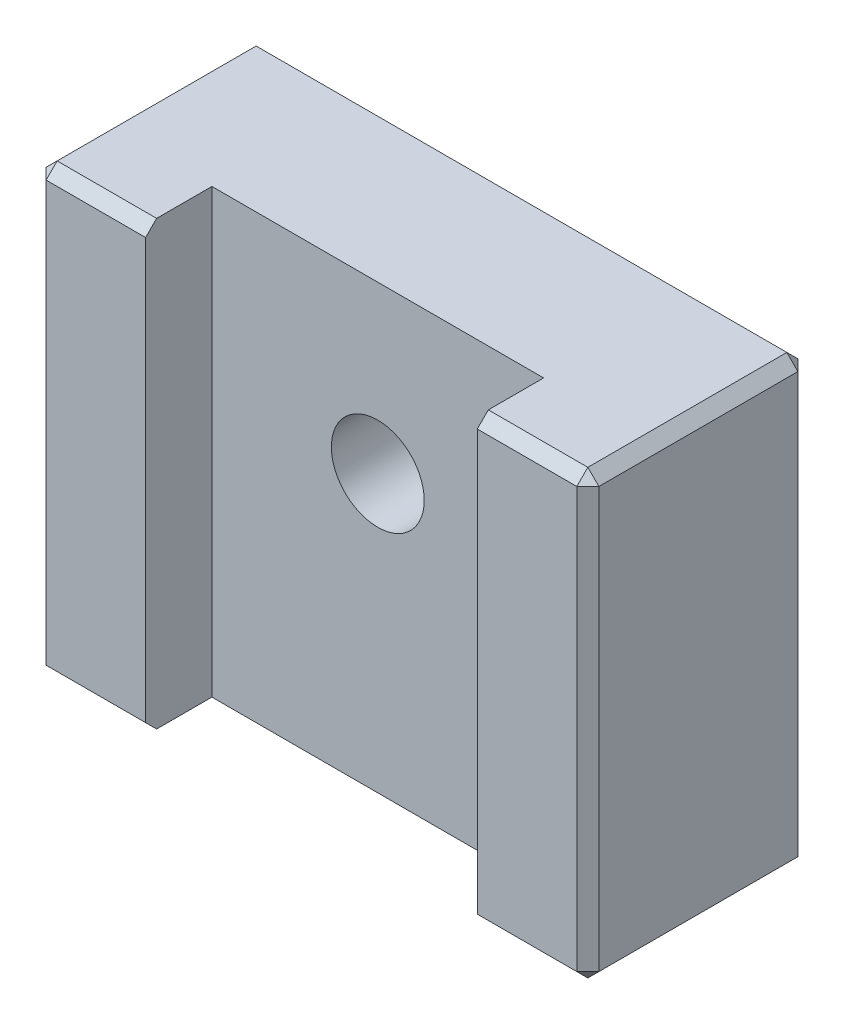
from build123d import *

# Parameters (mm, degrees)
SKETCH1_W             = 25
SKETCH1_H             = 20
BOSS_EXTRUDE1_DEPTH   = 10
SKETCH2_W             = 15
SKETCH2_H             = 20
CUT_EXTRUDE1_DEPTH    = 3
M5_TAPPED_HOLE1_D     = 4.2
M5_TAPPED_HOLE2_D     = 4.2
M5_TAPPED_HOLE2_DEPTH = 12.4
M5_TAPPED_HOLE2_TIP   = 1.2618073
CHAMFER1_SIZE         = 0.5


with BuildPart() as part:
    # Sketch1 → Boss-Extrude1 (new body)
    with BuildSketch(Plane.XY):
        Rectangle(SKETCH1_W, SKETCH1_H)
    extrude(amount=BOSS_EXTRUDE1_DEPTH)

    # Sketch2 → Cut-Extrude1 (cut)
    with BuildSketch(Plane.XY.offset(10)):
        Rectangle(SKETCH2_W, SKETCH2_H)
    extrude(amount=-CUT_EXTRUDE1_DEPTH, mode=Mode.SUBTRACT)

    # M5 Tapped Hole1 (through all)
    with Locations(Plane.XY.offset(7)):
        with Locations((0, 2.5)):
            Hole(M5_TAPPED_HOLE1_D / 2)

    # M5 Tapped Hole2
    with Locations(Plane(origin=(0, -10, 0), x_dir=(-1, 0, 0), z_dir=(0, -1, 0))):
        with Locations((8.5, -4), (-8.5, -4)):
            Hole(M5_TAPPED_HOLE2_D / 2, depth=M5_TAPPED_HOLE2_DEPTH)
            with Locations((0, 0, -(M5_TAPPED_HOLE2_DEPTH + M5_TAPPED_HOLE2_TIP / 2))):  # 118° drill point
                Cone(0, M5_TAPPED_HOLE2_D / 2, M5_TAPPED_HOLE2_TIP, mode=Mode.SUBTRACT)

    # Chamfer1
    chamfer1_edges = [part.edges().sort_by_distance(p)[0] for p in [
        (-12.5, 0, 10),
        (-10, -10, 10),
        (-10, 10, 10),
        (10, -10, 10),
        (12.5, 0, 10),
        (0, -10, 0),
        (-12.5, 0, 0),
        (0, 10, 0),
        (12.5, 0, 0),
        (10, 10, 10),
        (12.5, -10, 5),
        (-12.5, -10, 5),
        (-12.5, 10, 5),
        (12.5, 10, 5),
    ]]
    chamfer(chamfer1_edges, length=CHAMFER1_SIZE)


solid = part.part
